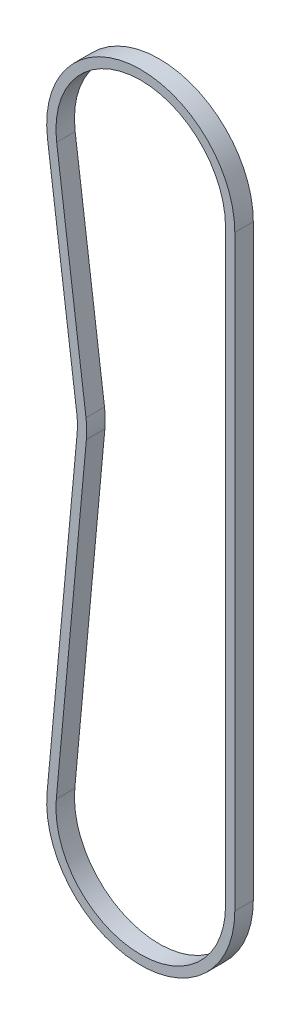
SolidWorks part; units mm, degrees
ref_plane "前视基准面" through (0, 0, 0) normal (0, 0, 1) x (1, 0, 0)
ref_plane "上视基准面" through (0, 0, 0) normal (0, 1, 0) x (1, 0, 0)
ref_plane "右视基准面" through (0, 0, 0) normal (1, 0, 0) x (0, 0, -1)
sketch "草图2" plane through (0, 0, 0) normal (0, 0, 1) x (1, 0, 0)
  line L0 (0, 0) -> (1, 0) construction
  line L1 (0, 0) -> (0, 1) construction
  line L2 (91.625, 0) -> (91.625, -635)
  line L3 (-91.2386, -626.5945) -> (-58.7614, -274.0676)
  line L4 (-59.1519, -253.7557) -> (-90.8481, -11.9063)
  arc A0 (-90.8481, -11.9063) -> (91.625, 0) centre (0, 0) cw
  arc A1 (91.625, -635) -> (-91.2386, -626.5945) centre (0, -635) cw
  arc A2 (-58.7614, -274.0676) -> (-59.1519, -253.7557) centre (-150, -265.6621) ccw
extrude "拉伸-薄壁1" add sketch "草图2" along normal mid plane 20 thin thin type one direction wall 10
